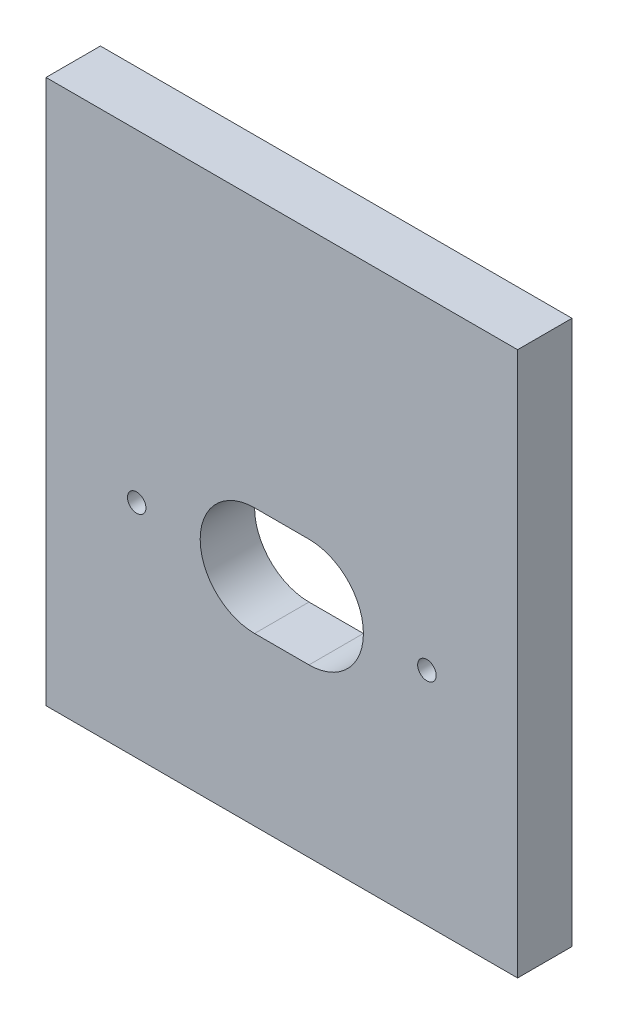
from build123d import *

# Parameters (mm, degrees)
SKETCH1_W            = 260
SKETCH1_H            = 300
BOSS_EXTRUDE1_DEPTH  = 30
M12_THREADED_HOLE1_D = 10.2


with BuildPart() as part:
    # Sketch1 → Boss-Extrude1 (new body)
    with BuildSketch(Plane.XY):
        with Locations((130, 150)):
            Rectangle(SKETCH1_W, SKETCH1_H)
        with BuildLine():
            Line((115, 152), (145, 152))
            ThreePointArc((145, 152), (175, 122), (145, 92))
            Line((145, 92), (115, 92))
            ThreePointArc((115, 92), (85, 122), (115, 152))
        make_face(mode=Mode.SUBTRACT)
    extrude(amount=BOSS_EXTRUDE1_DEPTH)

    # M12 Threaded hole1 (through all)
    with Locations(Plane(origin=(50, 122, 30), x_dir=(1, 0, 0), z_dir=(0, 0, 1))):
        with Locations((0, 0), (160, 0)):
            Hole(M12_THREADED_HOLE1_D / 2)


solid = part.part
